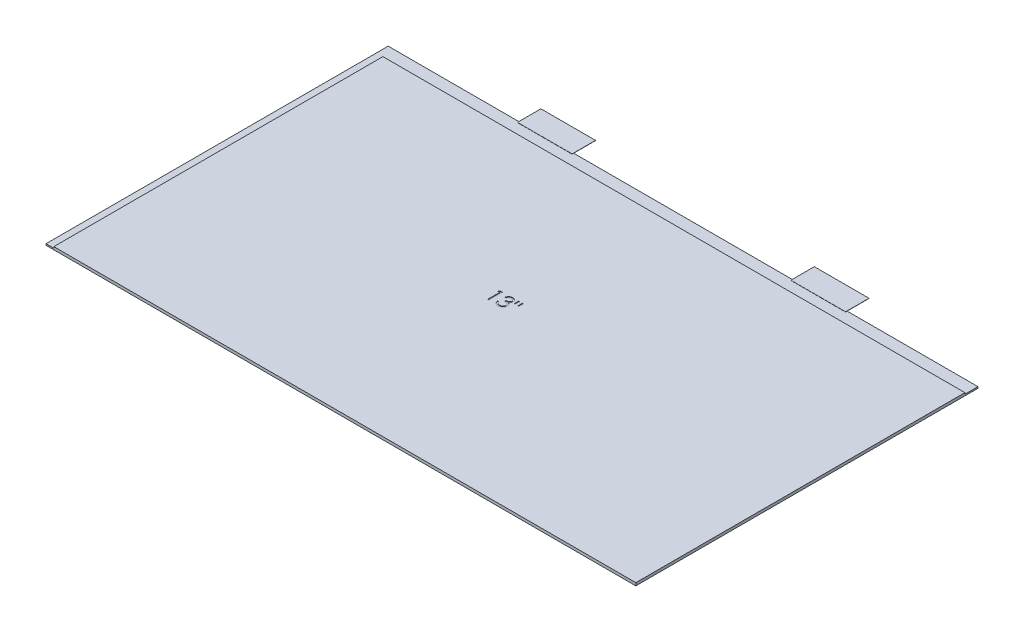
from build123d import *

# Parameters (mm, degrees)
SKETCH_2_W             = 301.97
SKETCH_2_H             = 175.19
BOSS_EXTRUDE_1_DEPTH   = 1.43
CUT_EXTRUDE_2_DEPTH    = 0.2
SKETCH_5_W             = 301.97
SKETCH_5_H             = 6.7
CUT_EXTRUDE_3_DEPTH    = 0.7
SKETCH_6_W             = 4
SKETCH_6_H             = 168.49
CUT_EXTRUDE_4_DEPTH    = 0.7
SKETCH_7_W             = 28
SKETCH_7_H             = 12
BOSS_EXTRUDE_2_DEPTH   = 0.1
LINEAR_PATTERN_1_COUNT = 2
LINEAR_PATTERN_1_PITCH = 140


with BuildPart() as part:
    # Sketch 2 → Boss-Extrude 1 (new body)
    with BuildSketch(Plane(origin=(0, 0, 0), x_dir=(1, 0, 0), z_dir=(0, 1, 0))):
        Rectangle(SKETCH_2_W, SKETCH_2_H)
    extrude(amount=BOSS_EXTRUDE_1_DEPTH)

    # Sketch 4 → Cut-Extrude 2 (cut)
    with BuildSketch(Plane(origin=(0, 1.43, 0), x_dir=(-1, 0, 0), z_dir=(0, 1, 0))):
        Polygon((13.229044249, -7.055555556), (11.924501425, -7.055555556), (11.924501425, 0), (12.557692308, 0), (12.557692308, -6.331908832), (13.643162393, -6.331908832), align=None)
        with BuildLine():
            Line((8.396723647, -5.427350427), (9.02991453, -5.427350427))
            add(Edge.make_bspline(
                [(9.02991453, -5.427350427), (9.012760356, -5.498374641), (8.97922535, -5.63722117), (8.909279448, -5.835597711), (8.833080949, -6.023322905), (8.741582278, -6.196881657), (8.641778917, -6.359761985), (8.527433113, -6.508269585), (8.403820339, -6.646181436), (8.267093854, -6.768571613), (8.123707504, -6.879399734), (7.97164089, -6.973893897), (7.813953469, -7.055182269), (7.649552709, -7.122150038), (7.477949157, -7.172598316), (7.300694202, -7.20920013), (7.117323336, -7.232969519), (6.992848035, -7.235289311), (6.929642984, -7.236467236)],
                knots=[0, 0, 0, 0, 1.162005537, 2.271625781, 3.343758855, 4.383309926, 5.390229558, 6.379919256, 7.361854164, 8.333198761, 9.295911338, 10.242430842, 11.177959212, 12.116337295, 13.062827104, 14.020064771, 14.994644689, 16, 16, 16, 16], degree=3))
            add(Edge.make_bspline(
                [(6.929642984, -7.236467236), (6.837552377, -7.233686883), (6.655379927, -7.228186825), (6.387746483, -7.177962485), (6.129660673, -7.098486424), (5.883947427, -6.988674308), (5.655713444, -6.853233216), (5.452642084, -6.692034461), (5.277485879, -6.50818825), (5.13054007, -6.305124192), (5.01548412, -6.088104355), (4.930643335, -5.864745308), (4.87899328, -5.63557689), (4.872299459, -5.480843962), (4.868945869, -5.403323095)],
                knots=[0, 0, 0, 0, 1.083050992, 2.142477498, 3.193116406, 4.255571735, 5.30263384, 6.308962982, 7.297363603, 8.282367274, 9.249857812, 10.179914175, 11.08814088, 12, 12, 12, 12], degree=3))
            add(Edge.make_bspline(
                [(4.868945869, -5.403323095), (4.871291521, -5.328722096), (4.875881597, -5.182739518), (4.914855893, -4.969618405), (4.980444867, -4.768753591), (5.071299785, -4.579299503), (5.188908942, -4.402457365), (5.331376125, -4.237829299), (5.499706887, -4.084685124), (5.627269191, -3.996955392), (5.692942041, -3.95178953)],
                knots=[0, 0, 0, 0, 1.024540389, 2.004866551, 2.965041327, 3.920577974, 4.882998113, 5.874504559, 6.905732034, 8, 8, 8, 8], degree=3))
            add(Edge.make_bspline(
                [(5.692942041, -3.95178953), (5.617791884, -3.915679202), (5.468656385, -3.844018249), (5.267429073, -3.701247147), (5.081971807, -3.540451451), (4.979761436, -3.413567658), (4.928307514, -3.349692842)],
                knots=[0, 0, 0, 0, 1.015663554, 2.015584519, 3.001021554, 4, 4, 4, 4], degree=3))
            add(Edge.make_bspline(
                [(4.928307514, -3.349692842), (4.894343687, -3.303216296), (4.826972214, -3.21102429), (4.744048511, -3.062711825), (4.667960424, -2.913246469), (4.611961795, -2.756751438), (4.563637197, -2.598253629), (4.53184122, -2.43435897), (4.511429475, -2.2666246), (4.508563249, -2.153097273), (4.507122507, -2.096031428)],
                knots=[0, 0, 0, 0, 1.02516404, 2.033540309, 3.025129118, 4.011046665, 4.991655828, 5.976607087, 6.982917762, 8, 8, 8, 8], degree=3))
            add(Edge.make_bspline(
                [(4.507122507, -2.096031428), (4.510748504, -1.997238489), (4.517983434, -1.800117531), (4.582372301, -1.508808314), (4.68281079, -1.224578162), (4.822788474, -0.951458), (4.996759546, -0.696697491), (5.202590989, -0.468099979), (5.44050197, -0.273396385), (5.70356555, -0.109273381), (5.989671277, 0.020792248), (6.294467942, 0.114515076), (6.616150937, 0.170735628), (6.83613539, 0.177481044), (6.948016827, 0.180911681)],
                knots=[0, 0, 0, 0, 0.955619592, 1.906742024, 2.874954321, 3.868585453, 4.869520953, 5.854611167, 6.836527075, 7.836578462, 8.849204403, 9.870874567, 10.917152508, 12, 12, 12, 12], degree=3))
            add(Edge.make_bspline(
                [(6.948016827, 0.180911681), (7.023444636, 0.179146208), (7.171861413, 0.175672345), (7.390134183, 0.152347175), (7.598044238, 0.10858745), (7.797610468, 0.053553541), (7.985820933, -0.022537006), (8.165382865, -0.113251033), (8.335509182, -0.220914784), (8.495189558, -0.345709317), (8.644253397, -0.485398135), (8.778903044, -0.642301861), (8.900628256, -0.813492126), (9.008655605, -1.000508816), (9.103439737, -1.202828123), (9.18294089, -1.421260777), (9.252355217, -1.654113393), (9.28469129, -1.81633906), (9.301282051, -1.89957265)],
                knots=[0, 0, 0, 0, 1.048603596, 2.063302207, 3.045874044, 3.999447474, 4.937100059, 5.862643889, 6.7929026, 7.7308982, 8.676022965, 9.627908155, 10.600123445, 11.591992905, 12.626222643, 13.701663232, 14.820785756, 16, 16, 16, 16], degree=3))
            Line((9.301282051, -1.89957265), (8.668091168, -1.89957265))
            add(Edge.make_bspline(
                [(8.668091168, -1.89957265), (8.651594692, -1.845246861), (8.619507612, -1.739578483), (8.564888948, -1.587500407), (8.502662431, -1.448086553), (8.435907686, -1.320314228), (8.365798755, -1.202925099), (8.287351208, -1.099023236), (8.206375312, -1.004044972), (8.145335981, -0.950534405), (8.115462518, -0.92434562)],
                knots=[0, 0, 0, 0, 1.198163088, 2.33053128, 3.407730985, 4.417276592, 5.372219308, 6.28897303, 7.162600585, 8, 8, 8, 8], degree=3))
            add(Edge.make_bspline(
                [(8.115462518, -0.92434562), (8.075953896, -0.893901696), (7.997058605, -0.833107821), (7.86857617, -0.755304947), (7.73297924, -0.688707547), (7.589137035, -0.634574389), (7.437030258, -0.593940088), (7.277275918, -0.56469343), (7.109611898, -0.545386092), (6.99518448, -0.543631615), (6.936709847, -0.542735043)],
                knots=[0, 0, 0, 0, 0.946083416, 1.889246487, 2.84504177, 3.809995578, 4.801312957, 5.829064617, 6.89060985, 8, 8, 8, 8], degree=3))
            add(Edge.make_bspline(
                [(6.936709847, -0.542735043), (6.870682051, -0.54397461), (6.741570396, -0.546398478), (6.553189754, -0.568753907), (6.373919013, -0.601169975), (6.205587632, -0.651875009), (6.045905032, -0.712704074), (5.898435792, -0.792340483), (5.758844497, -0.882276933), (5.631220527, -0.986890322), (5.516161278, -1.099966072), (5.416737374, -1.219929365), (5.330624903, -1.34306056), (5.261404846, -1.472232057), (5.206648533, -1.606176788), (5.169395221, -1.74539611), (5.143486475, -1.888717708), (5.141376871, -1.986142971), (5.14031339, -2.03525641)],
                knots=[0, 0, 0, 0, 1.216990249, 2.379719373, 3.493992396, 4.571561497, 5.616923107, 6.638958652, 7.655775068, 8.674704564, 9.676001865, 10.625896028, 11.54399481, 12.441854662, 13.322657739, 14.20572845, 15.095482574, 16, 16, 16, 16], degree=3))
            add(Edge.make_bspline(
                [(5.14031339, -2.03525641), (5.143404721, -2.100992598), (5.149571999, -2.232137879), (5.196462724, -2.42515422), (5.274281053, -2.611196599), (5.381105148, -2.787828631), (5.514259527, -2.949617204), (5.667449989, -3.094435416), (5.843945137, -3.215018861), (6.007310827, -3.298099277), (6.152391001, -3.353452476), (6.276296829, -3.392267861), (6.415137166, -3.423295429), (6.567243737, -3.453308702), (6.733258521, -3.478469851), (6.913330944, -3.499543322), (7.107533493, -3.516378915), (7.241974144, -3.523901348), (7.311253561, -3.527777778)],
                knots=[0, 0, 0, 0, 1.070440979, 2.135555593, 3.216243406, 4.345886539, 5.486149072, 6.621334998, 7.769144672, 8.957074012, 9.598644492, 10.297969361, 11.070758978, 11.915404831, 12.824182859, 13.805940418, 14.869366021, 16, 16, 16, 16], degree=3))
            Line((7.311253561, -3.527777778), (7.311253561, -4.251424501))
            add(Edge.make_bspline(
                [(7.311253561, -4.251424501), (7.223997859, -4.2531257), (7.05314514, -4.256456766), (6.802871441, -4.288448854), (6.564282395, -4.340376533), (6.340966734, -4.412874319), (6.138475327, -4.501134643), (5.96112159, -4.59995249), (5.815285861, -4.713954565), (5.698356211, -4.837751832), (5.611628219, -4.971370396), (5.547610738, -5.110003022), (5.509745747, -5.256228753), (5.504682015, -5.35600018), (5.502136752, -5.40614984)],
                knots=[0, 0, 0, 0, 1.321816535, 2.58820849, 3.816448615, 5.017641336, 6.139869627, 7.160068286, 8.085608132, 8.934319198, 9.728416342, 10.48890201, 11.240453369, 12, 12, 12, 12], degree=3))
            add(Edge.make_bspline(
                [(5.502136752, -5.40614984), (5.502953772, -5.443001672), (5.504579194, -5.516316646), (5.525896555, -5.623762669), (5.55644982, -5.727925506), (5.600837525, -5.827588083), (5.65824432, -5.923067217), (5.727697997, -6.014711631), (5.809374488, -6.103396446), (5.902743403, -6.187165723), (6.006945503, -6.262559555), (6.117798524, -6.329772106), (6.235734636, -6.386288293), (6.359985283, -6.433136374), (6.491222098, -6.468315377), (6.628754675, -6.493590721), (6.772865741, -6.509389136), (6.871183225, -6.511664059), (6.921162749, -6.512820513)],
                knots=[0, 0, 0, 0, 0.884246871, 1.759167212, 2.622361933, 3.489113179, 4.372562419, 5.294145153, 6.247651513, 7.265905295, 8.30305477, 9.334068495, 10.37719476, 11.441246459, 12.52060732, 13.637552802, 14.799054011, 16, 16, 16, 16], degree=3))
            add(Edge.make_bspline(
                [(6.921162749, -6.512820513), (7.001501306, -6.510021144), (7.158421193, -6.504553326), (7.384595228, -6.456493672), (7.59463756, -6.380348103), (7.754647447, -6.288402555), (7.873004885, -6.197952768), (7.959203557, -6.120138816), (8.042307907, -6.031913732), (8.119056845, -5.930857602), (8.194049328, -5.820445336), (8.266569293, -5.700068826), (8.334287394, -5.568011861), (8.375508512, -5.475145598), (8.396723647, -5.427350427)],
                knots=[0, 0, 0, 0, 1.4727372, 2.876598283, 4.222346151, 5.558423782, 6.24313385, 6.953189256, 7.68715613, 8.463578749, 9.278833271, 10.135787152, 11.040551781, 12, 12, 12, 12], degree=3))
        make_face()
        Polygon((1.440104167, -5.065527066), (1.879663016, -5.065527066), (1.974358974, -7.236467236), (1.341168091, -7.236467236), align=None)
        Polygon((3.335436699, -5.065527066), (3.779235666, -5.065527066), (3.873931624, -7.236467236), (3.240740741, -7.236467236), align=None)
    extrude(amount=-CUT_EXTRUDE_2_DEPTH, mode=Mode.SUBTRACT)

    # Sketch 5 → Cut-Extrude 3 (cut)
    with BuildSketch(Plane(origin=(0, 1.43, 0), x_dir=(1, 0, 0), z_dir=(0, 1, 0))):
        with Locations((0, 84.245)):
            Rectangle(SKETCH_5_W, SKETCH_5_H)
    extrude(amount=-CUT_EXTRUDE_3_DEPTH, mode=Mode.SUBTRACT)

    # Sketch 6 → Cut-Extrude 4 (cut)
    with BuildSketch(Plane(origin=(0, 1.43, 0), x_dir=(1, 0, 0), z_dir=(0, 1, 0))):
        with Locations((-148.985, -3.35)):
            Rectangle(SKETCH_6_W, SKETCH_6_H)
    extrude(amount=-CUT_EXTRUDE_4_DEPTH, mode=Mode.SUBTRACT)

    # Sketch 7 → Boss-Extrude 2 (add)
    with BuildSketch(Plane(origin=(0, 0.73, 0), x_dir=(1, 0, 0), z_dir=(0, 1, 0))):
        with Locations((69.985, 92.795)):
            Rectangle(SKETCH_7_W, SKETCH_7_H)
    boss_extrude_2 = extrude(amount=BOSS_EXTRUDE_2_DEPTH)

    # Linear Pattern 1: Boss-Extrude 2 ×2
    with Locations(*[(-i * LINEAR_PATTERN_1_PITCH, 0, 0) for i in range(1, LINEAR_PATTERN_1_COUNT)]):
        add(boss_extrude_2)


solid = part.part
